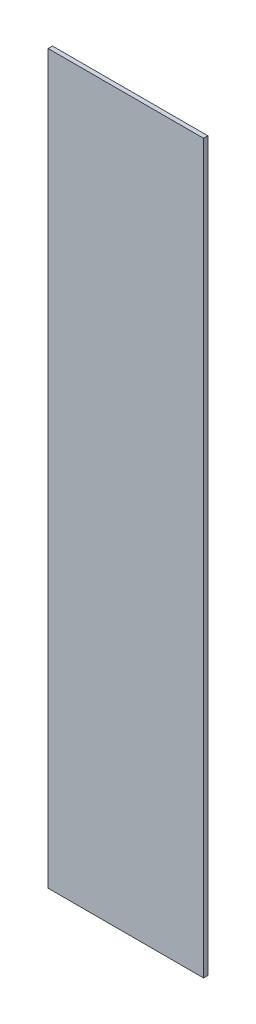
SolidWorks part; units mm, degrees
material "PMMA(有机玻璃)"
ref_plane "前视" through (0, 0, 0) normal (0, 0, 1) x (1, 0, 0)
ref_plane "上视" through (0, 0, 0) normal (0, 1, 0) x (1, 0, 0)
ref_plane "右视" through (0, 0, 0) normal (1, 0, 0) x (0, 0, -1)
sketch "草图1" plane through (0, 0, 0) normal (0, 0, 1) x (1, 0, 0)
  line L1 (-90, 421) -> (90, 421)
  line L2 (-90, 421) -> (-90, -421)
  line L3 (-90, -421) -> (90, -421)
  line L4 (90, 421) -> (90, -421)
  line L5 (-90, 421) -> (90, -421) construction
  line L6 (-90, -421) -> (90, 421) construction
  point P0 (0, 0)
  dimension "D1" = 842
  dimension "D2" = 180
extrude "凸台-拉伸1" add sketch "草图1" along normal blind 5
hole_wizard "M5 间隙孔1" positions "草图3" profile "草图2" hole size "M5" standard "GB"
sketch "草图3" plane through (0, 0, 5) normal (0, 0, 1) x (1, 0, 0)
  line L0 (-427.5, 273) -> (-427.5, -273) construction
  line L1 (-427.5, -273) -> (427.5, -273) construction
  line L2 (0, 273) -> (0, -273) construction
  line L3 (427.5, 273) -> (-427.5, 273) construction
  line L5 (-427.5, 0) -> (427.5, 0) construction
  line L6 (427.5, -273) -> (427.5, 273) construction
  point P0 (-375, -261)
  point P46 (415.5, 250)
  point P48 (-415.5, 250)
  point P58 (-125, -261)
  point P59 (125, -261)
  point P61 (-125, 261)
  point P62 (125, 261)
  point P64 (-375, 261)
  point P88 (375, -261)
  point P89 (375, 261)
  point P108 (415.5, 0)
  point P109 (-415.5, 0)
  point P110 (415.5, -250)
  point P111 (-415.5, -250)
  dimension "D1" = 12
  dimension "D2" = 12
  dimension "D5" = 3
  dimension "D3" = 12
  dimension "D6" = 4
  dimension "D4" = 2
sketch "草图2" plane through (-375, -261, 5) normal (1, 0, 0) x (0, -1, 0)
  line L0 (0, 0) -> (0, 5)
  line L1 (0, 5) -> (2.75, 5)
  line L2 (2.75, 5) -> (2.75, 0)
  line L5 (2.75, 0) -> (0, 0)
  line L11 (0, -6.35) -> (0, 107.95) construction
  dimension "通孔孔直径" = 5.5
  dimension "通孔孔深度" = 5
